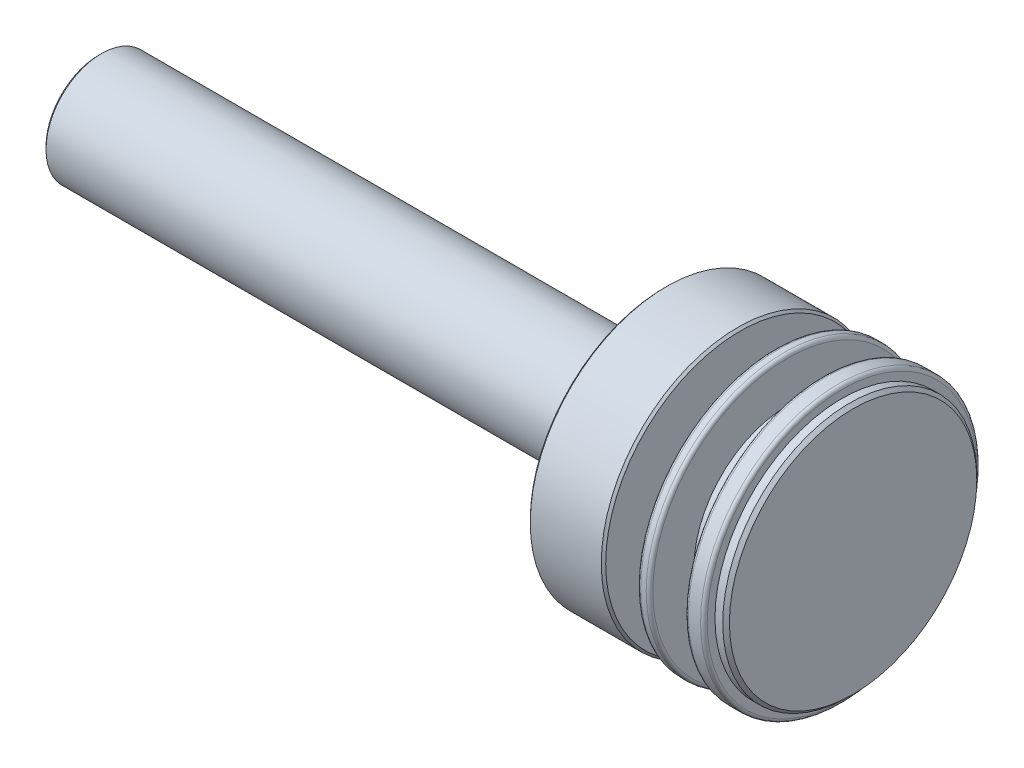
from build123d import *

# Parameters (mm, degrees)
M5_TAPPED_HOLE1_D     = 4.2
M5_TAPPED_HOLE1_DEPTH = 12.4
M5_TAPPED_HOLE1_TIP   = 1.2618073


with BuildPart() as part:
    # Sketch1 → Revolve1 (revolve)
    with BuildSketch(Plane.XY, mode=Mode.PRIVATE) as revolve1_sk:
        Polygon((-36, 0), (-36, 4.75), (-35.75, 5), (0, 5), (0, 0), align=None)
    revolve(revolve1_sk.sketch.rotate(Axis((0, 0, 0), (-1, 0, 0)), 270), axis=Axis((0, 0, 0), (-1, 0, 0)))

    # Sketch2 → Revolve2 (revolve)
    with BuildSketch(Plane.XY, mode=Mode.PRIVATE) as revolve2_sk:
        with BuildLine():
            Line((0, 0), (0, 5))
            Line((0, 5), (15, 5))
            Line((15, 5), (15, 12.1))
            Line((15, 12.1), (15.2, 12.3))
            Line((15.2, 12.3), (21.6, 12.3))
            Line((21.6, 12.3), (21.8, 12.1))
            Line((21.8, 12.1), (21.8, 6.5))
            Line((21.8, 6.5), (25, 6.5))
            Line((25, 6.5), (25, 12.15))
            ThreePointArc((25, 12.15), (25.087867966, 12.362132034), (25.3, 12.45))
            Line((25.3, 12.45), (25.8, 12.45))
            ThreePointArc((25.8, 12.45), (26.012132034, 12.362132034), (26.1, 12.15))
            Line((26.1, 12.15), (26.1, 8.45))
            Line((26.1, 8.45), (29.3, 8.45))
            Line((29.3, 8.45), (29.3, 12.15))
            ThreePointArc((29.3, 12.15), (29.387867966, 12.362132034), (29.6, 12.45))
            Line((29.6, 12.45), (30.7, 12.45))
            ThreePointArc((30.7, 12.45), (30.912132034, 12.362132034), (31, 12.15))
            Line((31, 12.15), (31, 11.45))
            Line((31, 11.45), (31.7, 11.45))
            Line((31.7, 11.45), (32, 11.15))
            Line((32, 11.15), (32, 0))
            Line((32, 0), (0, 0))
        make_face()
    revolve(revolve2_sk.sketch.rotate(Axis((32, 0, 0), (-1, 0, 0)), 270), axis=Axis((32, 0, 0), (-1, 0, 0)))

    # M5 Tapped Hole1
    with Locations(Plane.ZY.offset(36)):
        with Locations((0, 0)):
            Hole(M5_TAPPED_HOLE1_D / 2, depth=M5_TAPPED_HOLE1_DEPTH)
            with Locations((0, 0, -(M5_TAPPED_HOLE1_DEPTH + M5_TAPPED_HOLE1_TIP / 2))):  # 118° drill point
                Cone(0, M5_TAPPED_HOLE1_D / 2, M5_TAPPED_HOLE1_TIP, mode=Mode.SUBTRACT)


solid = part.part
